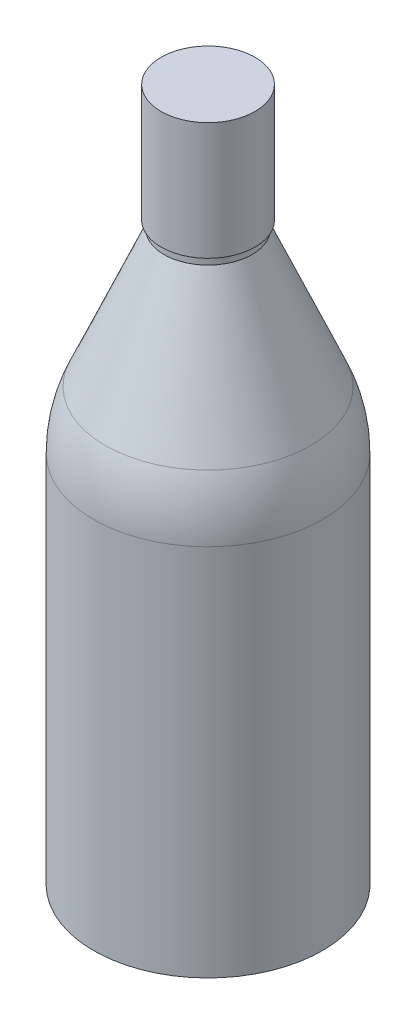
SolidWorks part; units mm, degrees
ref_plane "Front Plane" through (0, 0, 0) normal (0, 0, 1) x (1, 0, 0)
ref_plane "Top Plane" through (0, 0, 0) normal (0, 1, 0) x (1, 0, 0)
ref_plane "Right Plane" through (0, 0, 0) normal (1, 0, 0) x (0, 0, -1)
sketch "Sketch1" plane through (0, 0, 0) normal (0, 0, 1) x (1, 0, 0)
  line L0 (0, 0) -> (39, 0)
  line L1 (39, 0) -> (39, 127.1686)
  line L2 (7, 236) -> (15, 236)
  line L3 (0, 0) -> (0, 8)
  line L4 (15, 236) -> (15, 193.2909)
  line L5 (31, 8) -> (31, 135.8134)
  line L10 (8, 8) -> (8, 153.4718) construction
  line L13 (0, 0) -> (0, 285.072) construction
  line L14 (8, 153.4718) -> (8, 153.4718) construction
  line L15 (0, 236) -> (15, 236) construction
  line L16 (0, 0) -> (0, 236) construction
  line L18 (39, 139.7572) -> (15, 158.1834) construction
  line L19 (31, 135.8134) -> (8, 153.4718) construction
  line L21 (7, 236) -> (7, 191.6442)
  line L22 (8, 8) -> (31, 8) construction
  line L23 (0, 8) -> (31, 8)
  line L25 (15, 193.2909) -> (34.9356, 146.9149)
  line L27 (8, 153.4718) -> (8, 153.4718) construction
  line L28 (7, 191.6442) -> (31, 135.8134)
  line L29 (15, 236) -> (15, 158.1834) construction
  line L30 (39, 0) -> (39, 139.7572) construction
  arc A1 (39, 127.1686) -> (34.9356, 146.9149) centre (-11, 127.1686) ccw
  dimension "D5" = 50
  dimension "D7" = 30
  dimension "D1" = 39
  dimension "D2" = 236
  dimension "D3" = 8
  dimension "D4" = 8
  dimension "D6" = 8
revolve "Revolve1" add sketch "Sketch1" angle 360 about L3
sketch "Sketch2" plane through (0, 236, 0) normal (0, 1, 0) x (1, 0, 0)
  circle A0 centre (0, 0) radius 7 construction
  circle A1 centre (0, 0) radius 7
extrude "Boss-Extrude1" add sketch "Sketch2" against normal blind 5
ref_plane "Plane1" through (0, 196, 0) normal (0, 1, 0) x (1, 0, 0)
sketch "Sketch3" plane through (0, 196, 0) normal (0, 1, 0) x (1, 0, 0)
  circle A0 centre (0, 0) radius 16
  circle A1 centre (0, 0) radius 15 construction
  circle A2 centre (0, 0) radius 15
  dimension "D1" = 32
extrude "Boss-Extrude2" add sketch "Sketch3" along normal up to surface (40 mm away) up to face at (0, 236, -15)
